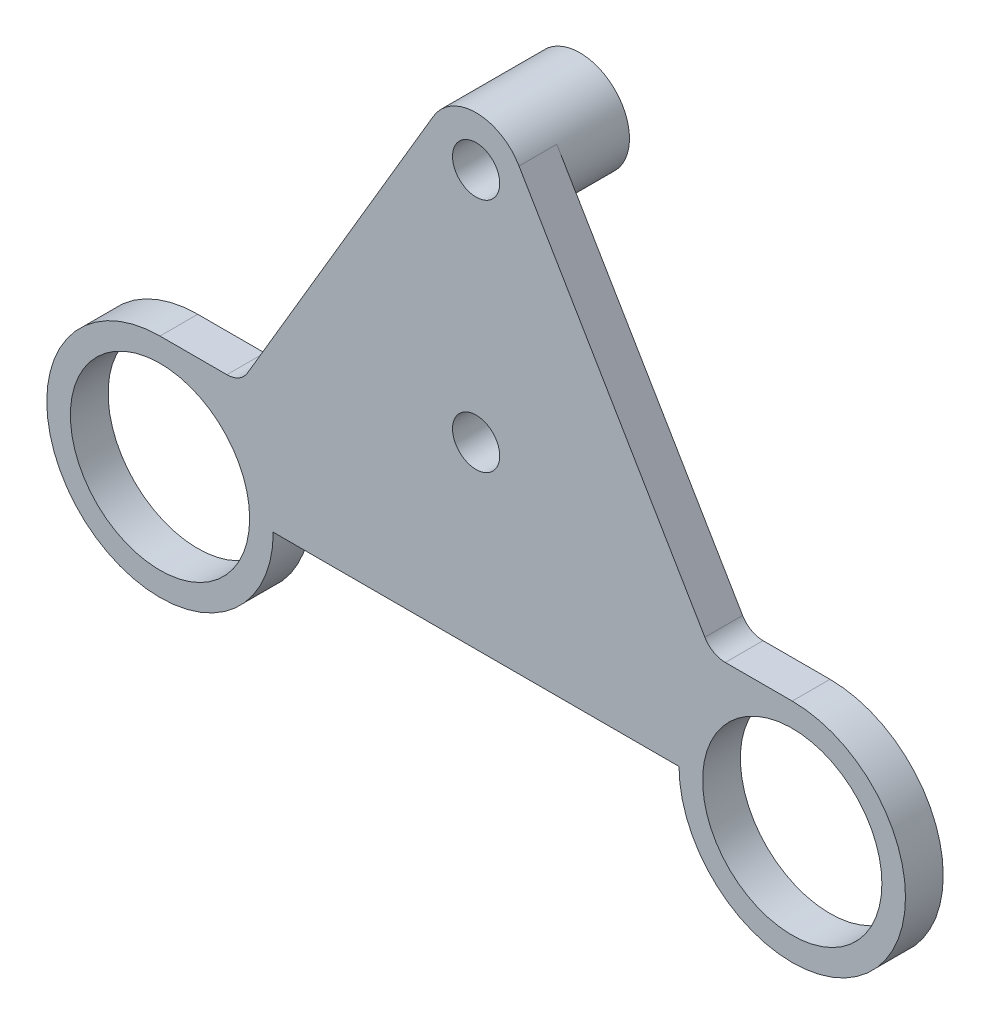
from build123d import *
from build123d.topology import SkipClean

# Parameters (mm, degrees)
SKETCH_1_R      = 19
SKETCH_1_R_2    = 5
EXTRUDE_1_DEPTH = 8
EXTRUDE_START   = 14
SKETCH_3_R      = 10.5
SKETCH_3_R_2    = 5
EXTRUDE_3_DEPTH = 14


with BuildPart() as part:
    # 草图1 → 凸台-拉伸1 (new body)
    with BuildSketch(Plane.XY):
        with BuildLine():
            ThreePointArc((-67, 24), (-83.970562748, -16.970562748), (-43, 0))
            Line((-43, 0), (43, 0))
            ThreePointArc((43, 0), (83.970562748, -16.970562748), (67, 24))
            Line((67, 24), (52.820062564, 24))
            ThreePointArc((52.820062564, 24), (50.319842999, 24.649533151), (48.477464605, 26.460232751))
            Line((48.477464605, 26.460232751), (9.09326674, 93.25))
            ThreePointArc((9.09326674, 93.25), (0, 98.5), (-9.09326674, 93.25))
            Line((-9.09326674, 93.25), (-48.477464605, 26.460232751))
            ThreePointArc((-48.477464605, 26.460232751), (-50.319842999, 24.649533151), (-52.820062564, 24))
            Line((-52.820062564, 24), (-67, 24))
        make_face()
        with Locations((-67, 0)):
            Circle(SKETCH_1_R, mode=Mode.SUBTRACT)
        with Locations((67, 0)):
            Circle(SKETCH_1_R, mode=Mode.SUBTRACT)
        with Locations((0, 38)):
            Circle(SKETCH_1_R_2, mode=Mode.SUBTRACT)
        with Locations((0, 88)):
            Circle(SKETCH_1_R_2, mode=Mode.SUBTRACT)
    extrude(amount=EXTRUDE_1_DEPTH)

    # 草图3 → 凸台-拉伸3 (add)
    # profile 1 of 2: a face of its own
    with SkipClean():  # the faces are left unmerged after this step: merging them gives an invalid solid
        with BuildSketch(Plane(origin=(0, 0, 0), x_dir=(-1, 0, 0), z_dir=(0, 0, -1)).offset(EXTRUDE_START)):
            with Locations((0, 88)):
                Circle(SKETCH_3_R)
            with Locations((0, 88)):
                Circle(SKETCH_3_R_2, mode=Mode.SUBTRACT)
        # profile 2 of 2: a face of its own
        with BuildSketch(Plane(origin=(0, 0, 0), x_dir=(-1, 0, 0), z_dir=(0, 0, -1)).offset(EXTRUDE_START)):
            with Locations(Location((0, 38, 0), (0, 0, 180))):
                Circle(SKETCH_3_R)
            with Locations((0, 38)):
                Circle(SKETCH_3_R_2, mode=Mode.SUBTRACT)
        extrude(amount=-EXTRUDE_3_DEPTH)


solid = part.part
